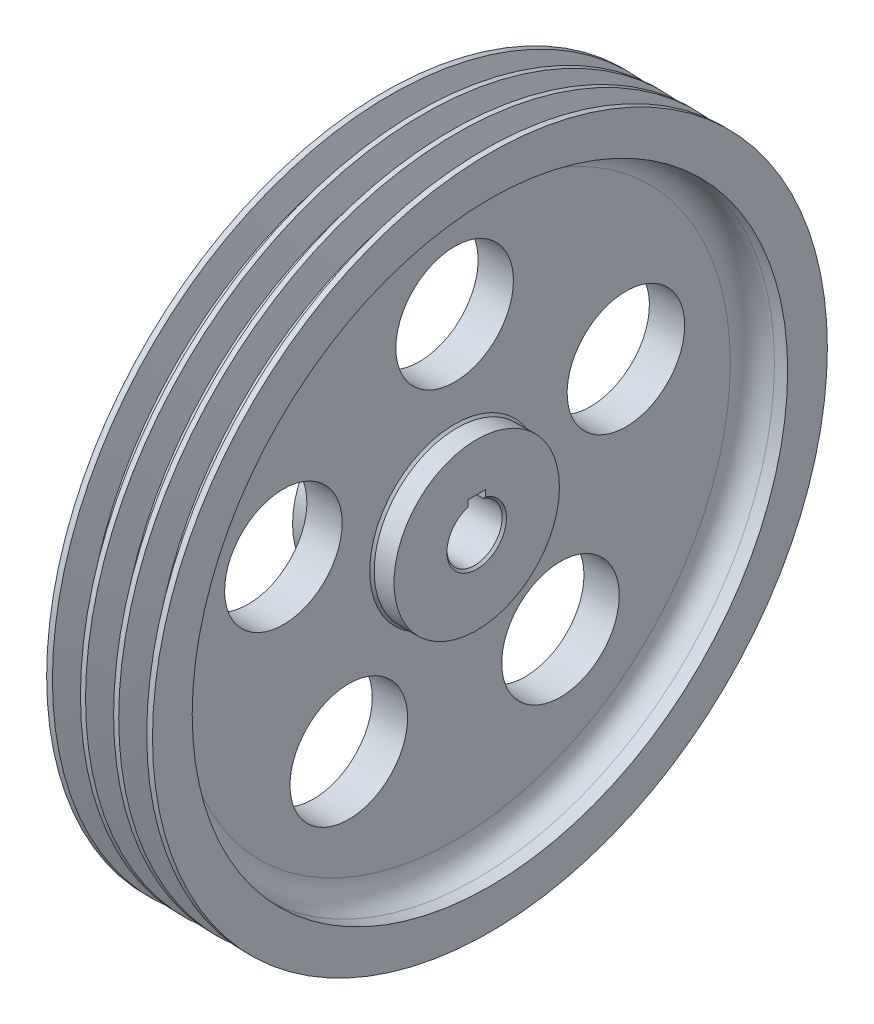
SolidWorks part; units mm, degrees
material "HT150"
ref_plane "Front Plane" through (0, 0, 0) normal (0, 0, 1) x (1, 0, 0)
ref_plane "Top Plane" through (0, 0, 0) normal (0, 1, 0) x (1, 0, 0)
ref_plane "Right Plane" through (0, 0, 0) normal (1, 0, 0) x (0, 0, -1)
sketch "Sketch1" plane through (0, 0, 0) normal (0, 0, 1) x (1, 0, 0)
  line L0 (6.1282, 141.5) -> (2.6123, 153)
  line L1 (2.6123, 153) -> (0, 153)
  line L2 (0, 153) -> (0, 12.5)
  line L3 (0, 12.5) -> (48, 12.5)
  line L4 (48, 12.5) -> (48, 153)
  line L5 (48, 153) -> (45.3877, 153)
  line L6 (45.3877, 153) -> (41.8718, 141.5)
  line L7 (41.8718, 141.5) -> (36.1918, 141.5)
  line L8 (36.1918, 141.5) -> (32.6759, 153)
  line L9 (32.6759, 153) -> (30.3559, 153)
  line L10 (30.3559, 153) -> (26.84, 141.5)
  line L11 (26.84, 141.5) -> (21.16, 141.5)
  line L12 (21.16, 141.5) -> (17.6441, 153)
  line L13 (17.6441, 153) -> (15.3241, 153)
  line L14 (15.3241, 153) -> (11.8082, 141.5)
  line L15 (11.8082, 141.5) -> (6.1282, 141.5)
  line L16 (0, 0) -> (61, 0) construction
  line L17 (8.9682, 141.5) -> (8.9682, 163.0492) construction
  line L18 (24, 141.5) -> (24, 147.3472) construction
  line L19 (39.0318, 141.5) -> (39.0318, 161.2464) construction
  point P24 (24, 12.5)
  dimension "D1" = 25
  dimension "D2" = 306
  dimension "D3" = 48
  dimension "D4" = 5.68
  dimension "D5" = 34
  dimension "D6" = 283
  dimension "D7" = 2.32
revolve "Revolve1" add sketch "Sketch1" angle 360 about L16
sketch "Sketch8" plane through (0, 0, 0) normal (-1, 0, 0) x (0, 0, 1)
  circle A0 centre (0, 0) radius 37.5
  circle A1 centre (0, 0) radius 12.5 construction
  circle A2 centre (0, 0) radius 12.5
  dimension "D1" = 75
extrude "Boss-Extrude2" add sketch "Sketch8" along normal blind 4
sketch "Sketch9" plane through (-4, 0, 0) normal (-1, 0, 0) x (0, 0, 1)
  line L0 (0, 0) -> (0, 12.5) construction
  line L1 (4, 15.8) -> (-4, 15.8)
  line L2 (4, 15.8) -> (4, 9.2)
  line L3 (4, 9.2) -> (-4, 9.2)
  line L4 (-4, 15.8) -> (-4, 9.2)
  line L5 (4, 15.8) -> (-4, 9.2) construction
  line L6 (4, 9.2) -> (-4, 15.8) construction
  circle A0 centre (0, 0) radius 12.5 construction
  point P0 (0, 12.5)
  dimension "D1" = 8
  dimension "D2" = 28.3
extrude "Cut-Extrude5" cut sketch "Sketch9" against normal up to next
sketch "Sketch10" plane through (0, 0, 0) normal (-1, 0, 0) x (0, 0, 1)
  circle A0 centre (0, 0) radius 135
  circle A1 centre (0, 0) radius 37.5 construction
  circle A2 centre (0, 0) radius 37.5
  dimension "D1" = 270
extrude "Cut-Extrude6" cut sketch "Sketch10" against normal blind 16
sketch "Sketch11" plane through (48, 0, 0) normal (1, 0, 0) x (0, 0, -1)
  circle A1 centre (0, 0) radius 37.5
  circle A2 centre (0, 0) radius 37.5
  circle A3 centre (0, 0) radius 135
  circle A4 centre (0, 0) radius 135
  dimension "D1" = 0
  dimension "D2" = 0
extrude "Cut-Extrude7" cut sketch "Sketch11" against normal blind 16
fillet "Fillet1" radius 10 2 edges at (16, 0, 135) (32, 0, -135)
chamfer "Chamfer1" distance 1 angle 45 2 edges at (32, 0, -37.5) (16, 0, 37.5)
sketch "Sketch13" plane through (48, 0, 0) normal (1, 0, 0) x (0, 0, -1)
  circle A1 centre (0, 0) radius 37.5
  circle A2 centre (0, 0) radius 37.5
  dimension "D1" = 0
extrude "Cut-Extrude9" cut sketch "Sketch13" against normal blind 6
chamfer "Chamfer2" distance 1 angle 45 2 edges at (-4, -12.5, 0) (42, -12.5, 0)
sketch "Sketch12" plane through (16, 0, 0) normal (-1, 0, 0) x (0, 0, 1)
  circle A0 centre (0, 0) radius 81.65 construction
  circle A1 centre (0, 81.65) radius 26.65
  dimension "D1" = 163.3
  dimension "D2" = 53.3
extrude "Cut-Extrude8" cut sketch "Sketch12" against normal up to next
pattern_circular "CirPattern1" count 5 over 360 about axis through (0, 0, 0) along (1, 0, 0) of "Cut-Extrude8"
